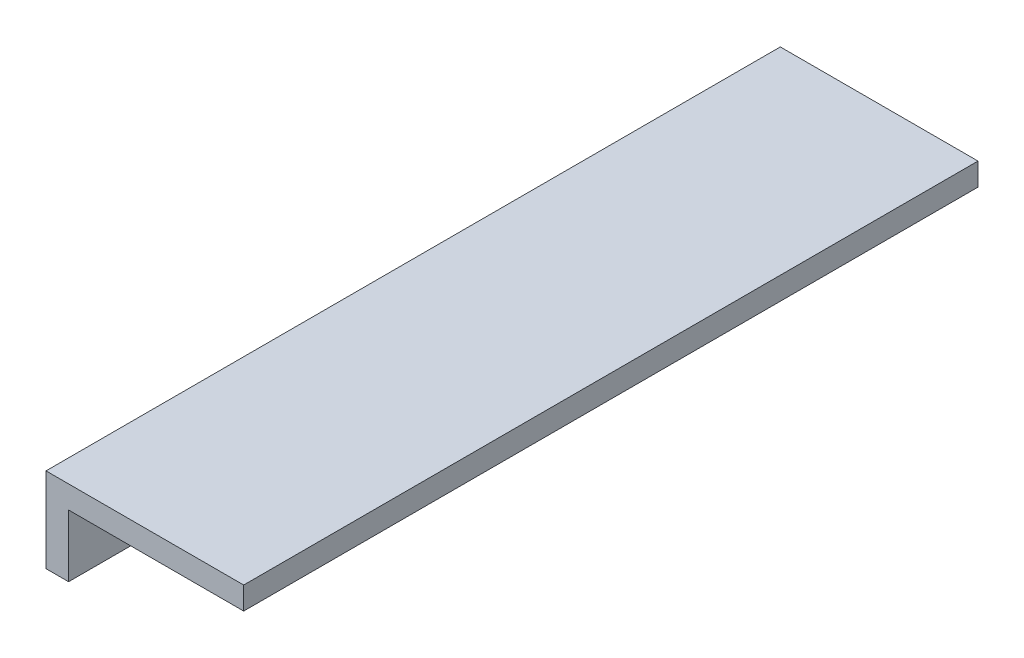
SolidWorks part; units mm, degrees
ref_plane "前视基准面" through (0, 0, 0) normal (0, 0, 1) x (1, 0, 0)
ref_plane "上视基准面" through (0, 0, 0) normal (0, 1, 0) x (1, 0, 0)
ref_plane "右视基准面" through (0, 0, 0) normal (1, 0, 0) x (0, 0, -1)
sketch "草图1" plane through (0, 0, 0) normal (0, 0, 1) x (1, 0, 0)
  line L0 (0, 0) -> (70, 0)
  line L1 (0, 0) -> (0, -30)
  line L2 (8, -8) -> (8, -30)
  line L3 (8, -8) -> (70, -8)
  line L4 (70, -8) -> (70, 0)
  line L5 (0, -30) -> (8, -30)
  dimension "D1" = 8
extrude "凸台-拉伸1" add sketch "草图1" along normal blind 260
sketch "草图2" plane through (0, 0, 0) normal (-1, 0, 0) x (0, 0, 1)
  line L0 (260, -30) -> (210, -30)
  line L1 (260, -30) -> (0, -30) construction
  line L2 (210, -30) -> (210, -15)
  line L3 (210, -15) -> (160, -15)
  line L4 (160, -15) -> (160, -30)
  line L5 (160, -30) -> (210, -30)
  line M2 (0, -30) -> (260, -30)
extrude "切除-拉伸1" cut sketch "草图2" against normal blind 10 contours L3 L4 L2 M2
